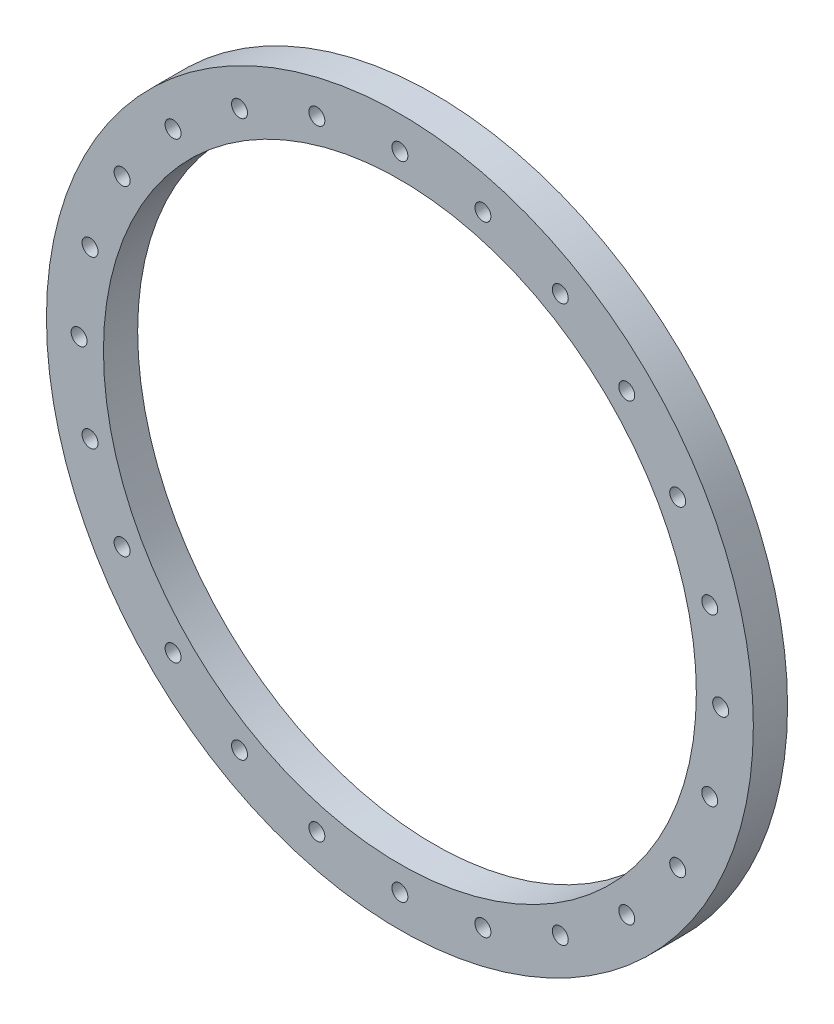
from build123d import *

# Parameters (mm, degrees)
SKETCH1_R               = 465
SKETCH1_R_2             = 390
BOSS_EXTRUDE1_DEPTH     = 45
M24_THREADED_HOLE1_D    = 21
CIRCULAR_PATTERN1_COUNT = 24


with BuildPart() as part:
    # Sketch1 → Boss-Extrude1 (new body)
    with BuildSketch(Plane.XY):
        with Locations(Location((0, 0, 0), (0, 0, 180))):
            Circle(SKETCH1_R)
        with Locations(Location((0, 0, 0), (0, 0, 180))):
            Circle(SKETCH1_R_2, mode=Mode.SUBTRACT)
    extrude(amount=BOSS_EXTRUDE1_DEPTH)

    # M24 Threaded hole1 (through all)
    with Locations(Plane(origin=(-422, 0, 45), x_dir=(1, 0, 0), z_dir=(0, 0, 1))):
        with Locations((0, 0)):
            m24_threaded_hole1 = Hole(M24_THREADED_HOLE1_D / 2)

    # Circular pattern1: M24 Threaded hole1 ×24 about axis
    circular_pattern1_axis = Axis((0, 0, 0), (0, 0, 1))
    for i in range(1, CIRCULAR_PATTERN1_COUNT):
        add(m24_threaded_hole1.rotate(circular_pattern1_axis, i * 360 / CIRCULAR_PATTERN1_COUNT), mode=Mode.SUBTRACT)


solid = part.part
